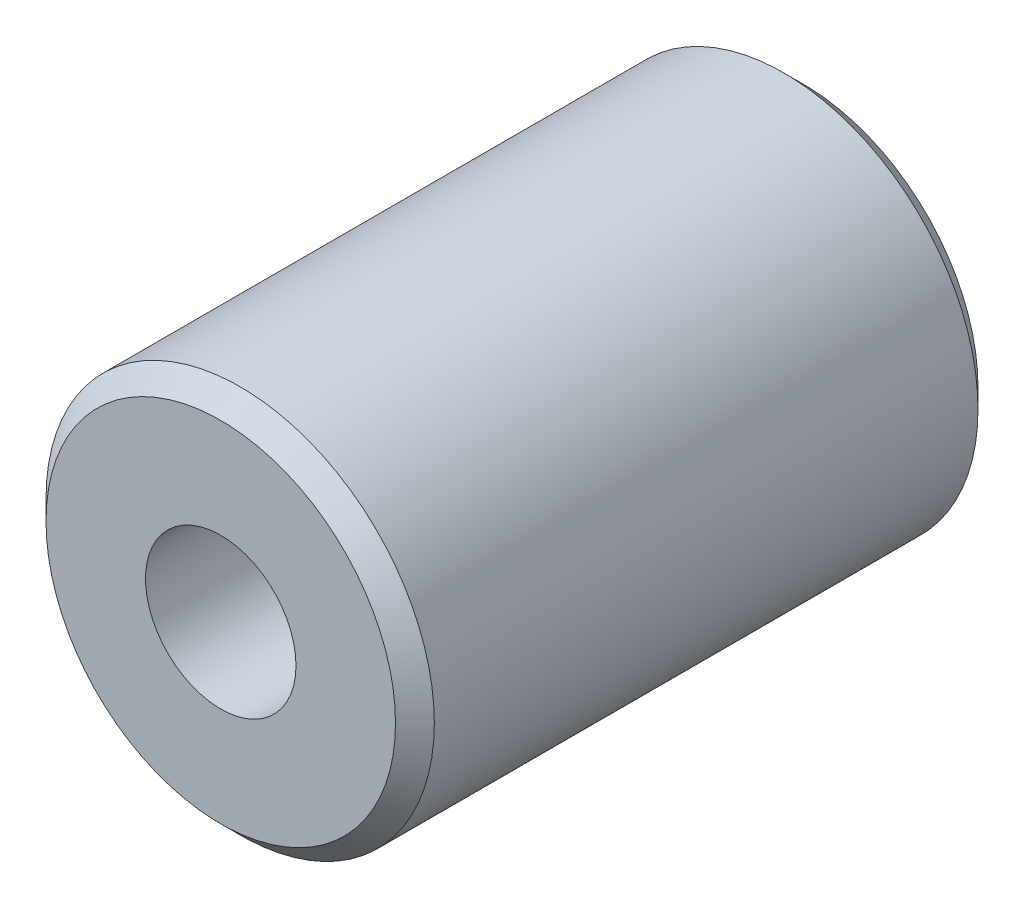
from build123d import *

# Parameters (mm, degrees)
SKETCH1_R           = 20
BOSS_EXTRUDE1_DEPTH = 30
CHAMFER1_SIZE       = 2
M18_TAPPED_HOLE1_D  = 15.5


with BuildPart() as part:
    # Sketch1 → Boss-Extrude1 (new, symmetric)
    with BuildSketch(Plane.XY):
        Circle(SKETCH1_R)
    extrude(amount=BOSS_EXTRUDE1_DEPTH, both=True)

    # Chamfer1
    chamfer1_edges = [part.edges().sort_by_distance(p)[0] for p in [
        (-20, 0, -30),
        (-20, 0, 30),
    ]]
    chamfer(chamfer1_edges, length=CHAMFER1_SIZE)

    # M18 Tapped Hole1 (through all)
    with Locations(Plane.XY.offset(30)):
        with Locations((0, 0)):
            Hole(M18_TAPPED_HOLE1_D / 2)


solid = part.part
